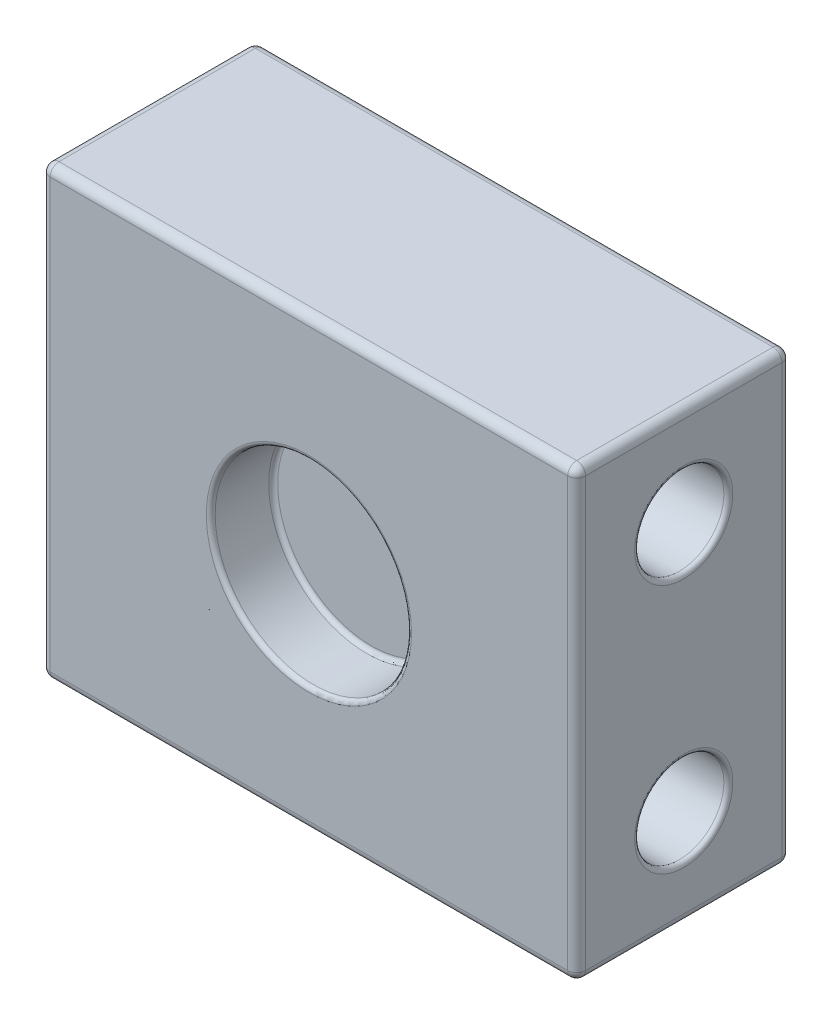
SolidWorks part; units mm, degrees
material "ABS PC"
ref_plane "Front Plane" through (0, 0, 0) normal (0, 0, 1) x (1, 0, 0)
ref_plane "Top Plane" through (0, 0, 0) normal (0, 1, 0) x (1, 0, 0)
ref_plane "Right Plane" through (0, 0, 0) normal (1, 0, 0) x (0, 0, -1)
sketch "Sketch1" plane through (0, 0, 0) normal (0, 0, 1) x (1, 0, 0)
  line L1 (30, -25) -> (-30, -25)
  line L2 (30, -25) -> (30, 25)
  line L3 (30, 25) -> (-30, 25)
  line L4 (-30, -25) -> (-30, 25)
  line L5 (30, -25) -> (-30, 25) construction
  line L6 (30, 25) -> (-30, -25) construction
  point P0 (0, 0)
  dimension "D1" = 60
  dimension "D2" = 50
extrude "Boss-Extrude1" add sketch "Sketch1" along normal mid plane 24
sketch "Sketch2" plane through (0, 0, 12) normal (0, 0, 1) x (1, 0, 0)
  circle A0 centre (0, 0) radius 11
  dimension "D1" = 22
extrude "Cut-Extrude1" cut sketch "Sketch2" against normal blind 7
sketch "Sketch3" plane through (30, 0, 0) normal (1, 0, 0) x (0, 0, -1)
  line L0 (0, 0) -> (17.8239, 0) construction
  circle A0 centre (0, 14) radius 5
  circle A1 centre (0, -14) radius 5
  dimension "D1" = 28
  dimension "D2" = 10
extrude "Cut-Extrude2" cut sketch "Sketch3" against normal through all
fillet "Fillet1" radius 1 12 edges at (-30, -25, 0) (0, -25, 12) (30, -25, 0) (0, -25, -12) (30, 25, 0) (0, 25, 12) (-30, 25, 0) (0, 25, -12) (-30, 0, -12) (30, 0, -12) (-30, 0, 12) (30, 0, 12)
fillet "Fillet2" radius 0.5 6 edges at (11, 0, 12) (11, 0, 5) (30, -14, -5) (-30, -14, -5) (30, 14, -5) (-30, 14, -5)
